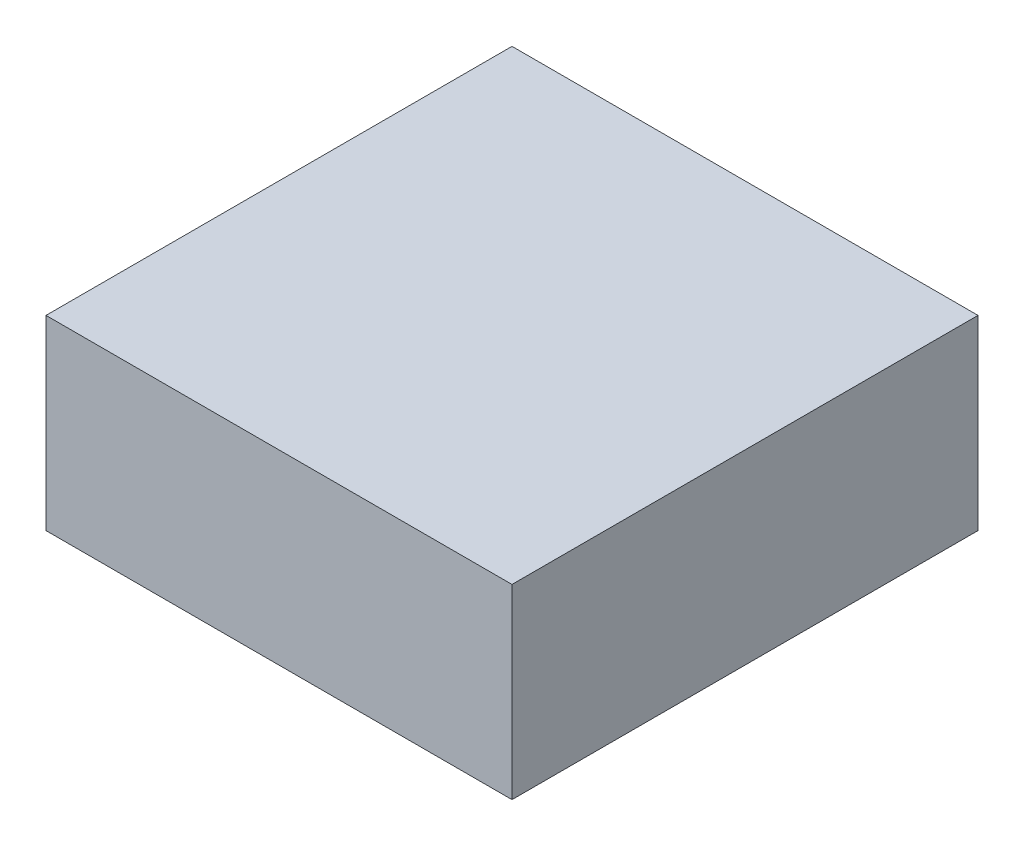
SolidWorks part; units mm, degrees
ref_plane "Front Plane" through (0, 0, 0) normal (0, 0, 1) x (1, 0, 0)
ref_plane "Top Plane" through (0, 0, 0) normal (0, 1, 0) x (1, 0, 0)
ref_plane "Right Plane" through (0, 0, 0) normal (1, 0, 0) x (0, 0, -1)
sketch "Sketch1" plane through (0, 0, 0) normal (0, 1, 0) x (1, 0, 0)
  line L1 (-75, 75) -> (75, 75)
  line L2 (-75, 75) -> (-75, -75)
  line L3 (-75, -75) -> (75, -75)
  line L4 (75, 75) -> (75, -75)
  line L5 (-75, 75) -> (75, -75) construction
  line L6 (-75, -75) -> (75, 75) construction
  point P0 (0, 0)
  dimension "D1" = 150
  dimension "D2" = 150
extrude "Boss-Extrude1" add sketch "Sketch1" along normal blind 60
